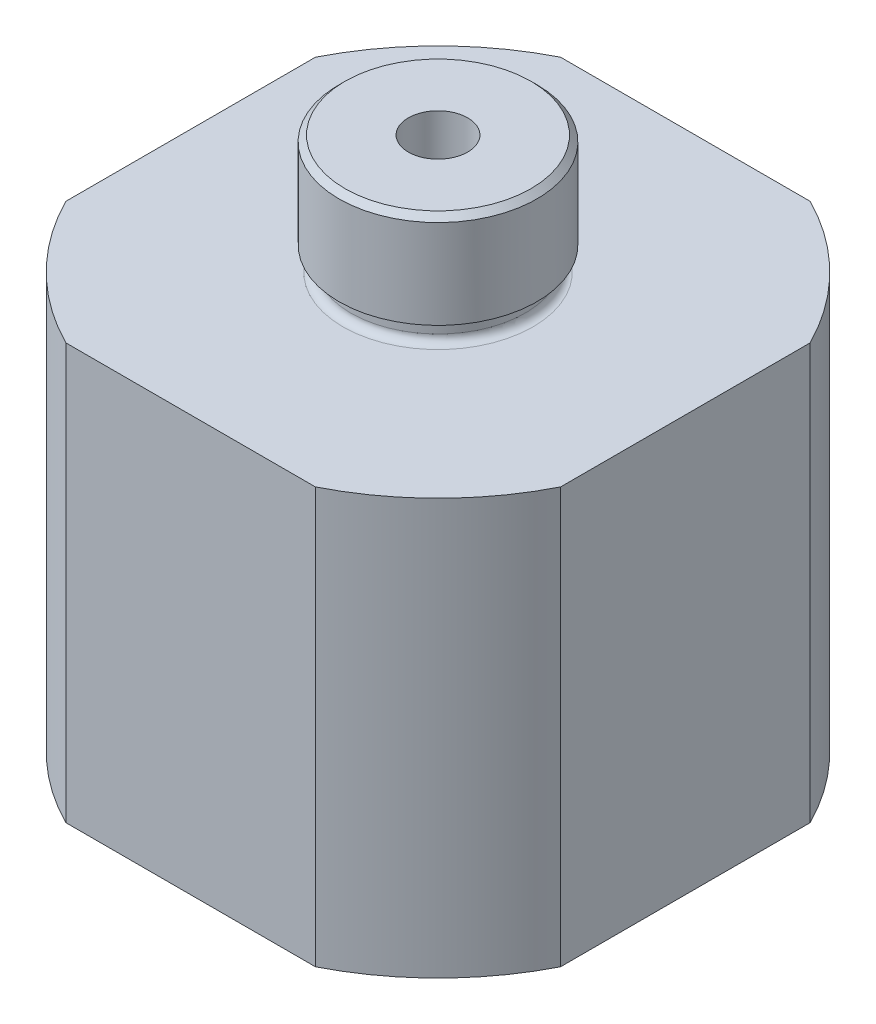
from build123d import *

# Parameters (mm, degrees)
FILLET1_R           = 0.4
SKETCH2_R           = 10
CUT_EXTRUDE1_DEPTH  = 14
SKETCH3_R           = 10.25
CUT_EXTRUDE2_DEPTH  = 4
SKETCH4_R           = 1.5
CUT_EXTRUDE3_DEPTH  = 90
CHAMFER1_SIZE       = 0.3
CHAMFER2_SIZE       = 1
SKETCH5_OUTSIDE_W   = 39.586
SKETCH5_OUTSIDE_H   = 39.586
SKETCH5_OUTSIDE_W_2 = 25
SKETCH5_OUTSIDE_H_2 = 25
CUT_EXTRUDE4_DEPTH  = 90


with BuildPart() as part:
    # Sketch1 → Revolve1 (revolve)
    with BuildSketch(Plane.XY, mode=Mode.PRIVATE) as revolve1_sk:
        Polygon((0, 0), (-14, 0), (-14, 21), (-4.4, 21), (-4.4, 22.2), (-5, 22.2), (-5, 27), (0, 27), align=None)
    revolve(revolve1_sk.sketch.rotate(Axis((0, 27, 0), (0, -1, 0)), 270), axis=Axis((0, 27, 0), (0, -1, 0)))

    # Fillet1
    fillet1_edges = [part.edges().sort_by_distance(p)[0] for p in [
        (0, 22.2, -4.4),
        (0, 21, -4.4),
    ]]
    fillet(fillet1_edges, radius=FILLET1_R)

    # Sketch2 → Cut-Extrude1 (cut)
    with BuildSketch(Plane.XZ):
        with Locations(Location((0, 0, 0), (0, 0, 270))):
            Circle(SKETCH2_R)
    extrude(amount=-CUT_EXTRUDE1_DEPTH, mode=Mode.SUBTRACT)

    # Sketch3 → Cut-Extrude2 (cut)
    with BuildSketch(Plane.XZ.offset(-14)):
        with Locations(Location((0, 0, 0), (0, 0, 270))):
            Circle(SKETCH3_R)
    extrude(amount=-CUT_EXTRUDE2_DEPTH, mode=Mode.SUBTRACT)

    # Sketch4 → Cut-Extrude3 (cut)
    with BuildSketch(Plane.XZ.offset(-18)):
        with Locations(Location((0, 0, 0), (0, 0, 270))):
            Circle(SKETCH4_R)
    extrude(amount=-CUT_EXTRUDE3_DEPTH, mode=Mode.SUBTRACT)

    # Chamfer1
    chamfer1_edges = [part.edges().sort_by_distance(p)[0] for p in [
        (0, 27, -5),
    ]]
    chamfer(chamfer1_edges, length=CHAMFER1_SIZE)

    # Chamfer2
    chamfer2_edges = [part.edges().sort_by_distance(p)[0] for p in [
        (0, 0, 10),
    ]]
    chamfer(chamfer2_edges, length=CHAMFER2_SIZE)

    # Sketch5 outside → Cut-Extrude4 (cut)
    with BuildSketch(Plane(origin=(0, 21, 0), x_dir=(1, 0, 0), z_dir=(0, 1, 0))):
        Rectangle(SKETCH5_OUTSIDE_W, SKETCH5_OUTSIDE_H)
        Rectangle(SKETCH5_OUTSIDE_W_2, SKETCH5_OUTSIDE_H_2, mode=Mode.SUBTRACT)
    extrude(amount=-CUT_EXTRUDE4_DEPTH, mode=Mode.SUBTRACT)


solid = part.part
